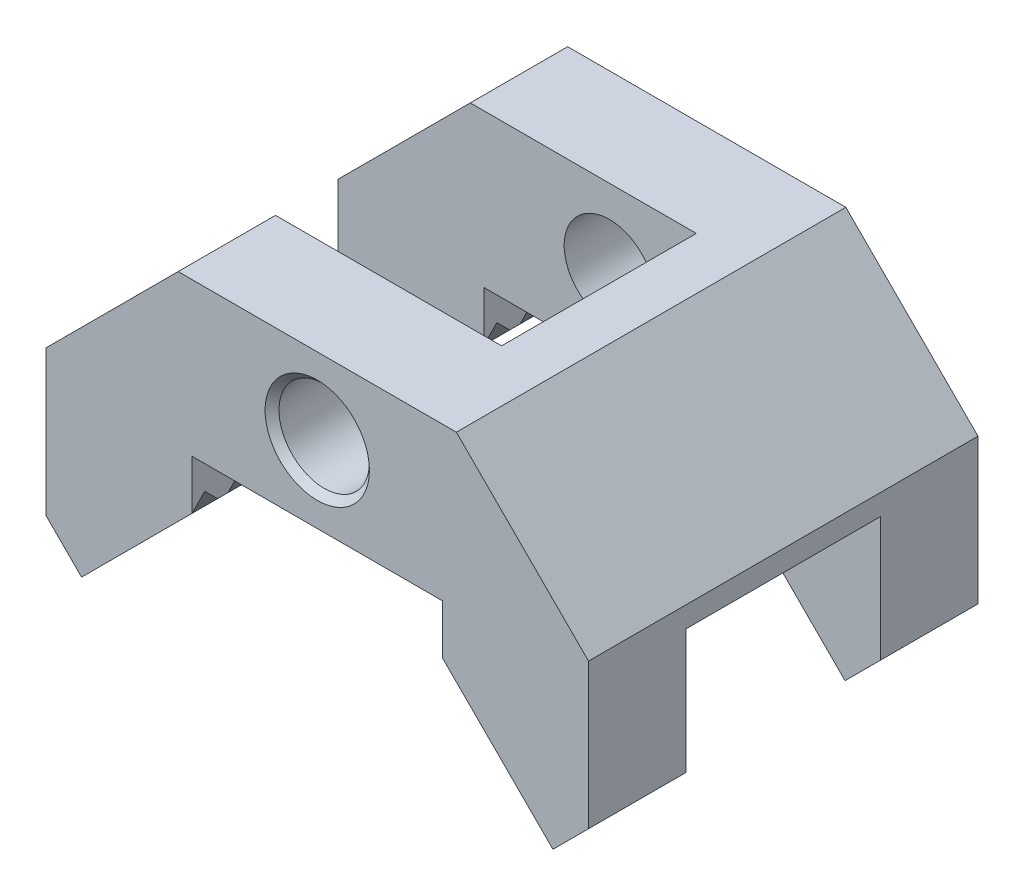
from build123d import *

# Parameters (mm, degrees)
SKETCH1_R            = 6.5
BOSS_EXTRUDE1_DEPTH  = 28
CUT_EXTRUDE1_START   = -14
SKETCH2_W            = 65.403152184
SKETCH2_H            = 73.649752858
CUT_EXTRUDE1_DEPTH   = 28
CUT_EXTRUDE2_DEPTH   = 28
MIRROR2_COPY_1_DEPTH = 28
CHAMFER1_SIZE        = 1
CUT_EXTRUDE3_START   = -14
SKETCH6_W            = 28.147073634
SKETCH6_H            = 26.396452471
CUT_EXTRUDE3_DEPTH   = 28


with BuildPart() as part:
    # Sketch1 → Boss-Extrude1 (new, symmetric)
    with BuildSketch(Plane.XY):
        Polygon((20, 11), (-20, 11), (-39, -8), (-39, -28.882250994), (-33.884776311, -33.997474683), (-18, -18.112698372), (-18, -11), (18, -11), (18, -18.112698372), (33.884776311, -33.997474683), (39, -28.882250994), (39, -8), align=None)
        Circle(SKETCH1_R, mode=Mode.SUBTRACT)
    extrude(amount=BOSS_EXTRUDE1_DEPTH, both=True)

    # Sketch2 → Cut-Extrude1 (cut)
    with BuildSketch(Plane.XY.offset(28).offset(CUT_EXTRUDE1_START)):
        with Locations((-20.201576092, 0)):
            Rectangle(SKETCH2_W, SKETCH2_H)
    extrude(amount=-CUT_EXTRUDE1_DEPTH, mode=Mode.SUBTRACT)

    # Sketch5 → Cut-Extrude2 (cut)
    with BuildSketch(Plane(origin=(-33.941125497, -33.941125497, 0), x_dir=(0, 0, 1), z_dir=(-0.7071067811865506, -0.7071067811865445, 0))):
        Polygon((-22.833333333, -0.079689783), (-19.166666667, -0.079689783), (-21, 1.216672649), align=None)
        Polygon((-17.666666667, -0.079689783), (-14, -0.079689783), (-15.833333333, 1.216672649), align=None)
        Polygon((-24.333333333, -0.079689783), (-26.166666667, 1.216672649), (-28, -0.079689783), align=None)
    cut_extrude2 = extrude(amount=-CUT_EXTRUDE2_DEPTH, mode=Mode.SUBTRACT)

    # Mirror1: Cut-Extrude2 across plane
    add(cut_extrude2.mirror(Plane.XY), mode=Mode.SUBTRACT)

    # Mirror2: Cut-Extrude2 across plane
    add(cut_extrude2.mirror(Plane(origin=(0, 0, 0), x_dir=(0, 0, 1), z_dir=(1, 0, 0))), mode=Mode.SUBTRACT)

    # Mirror2 copy 1 sketch → Mirror2 copy 1 (cut)
    with BuildSketch(Plane(origin=(33.941125497, -33.941125497, 0), x_dir=(0, 0, -1), z_dir=(0.7071067811865506, -0.7071067811865445, 0))):
        Polygon((-22.833333333, -0.079689783), (-19.166666667, -0.079689783), (-21, 1.216672649), align=None)
        Polygon((-17.666666667, -0.079689783), (-14, -0.079689783), (-15.833333333, 1.216672649), align=None)
        Polygon((-24.333333333, -0.079689783), (-26.166666667, 1.216672649), (-28, -0.079689783), align=None)
    extrude(amount=-MIRROR2_COPY_1_DEPTH, mode=Mode.SUBTRACT)

    # Chamfer1
    chamfer1_edges = [part.edges().sort_by_distance(p)[0] for p in [
        (-6.5, 0, -28),
        (-6.5, 0, 28),
    ]]
    chamfer(chamfer1_edges, length=CHAMFER1_SIZE)

    # Sketch6 → Cut-Extrude3 (cut)
    with BuildSketch(Plane.XY.offset(28).offset(CUT_EXTRUDE3_START)):
        with Locations((32.073536817, -24.198226236)):
            Rectangle(SKETCH6_W, SKETCH6_H)
    extrude(amount=-CUT_EXTRUDE3_DEPTH, mode=Mode.SUBTRACT)


solid = part.part
